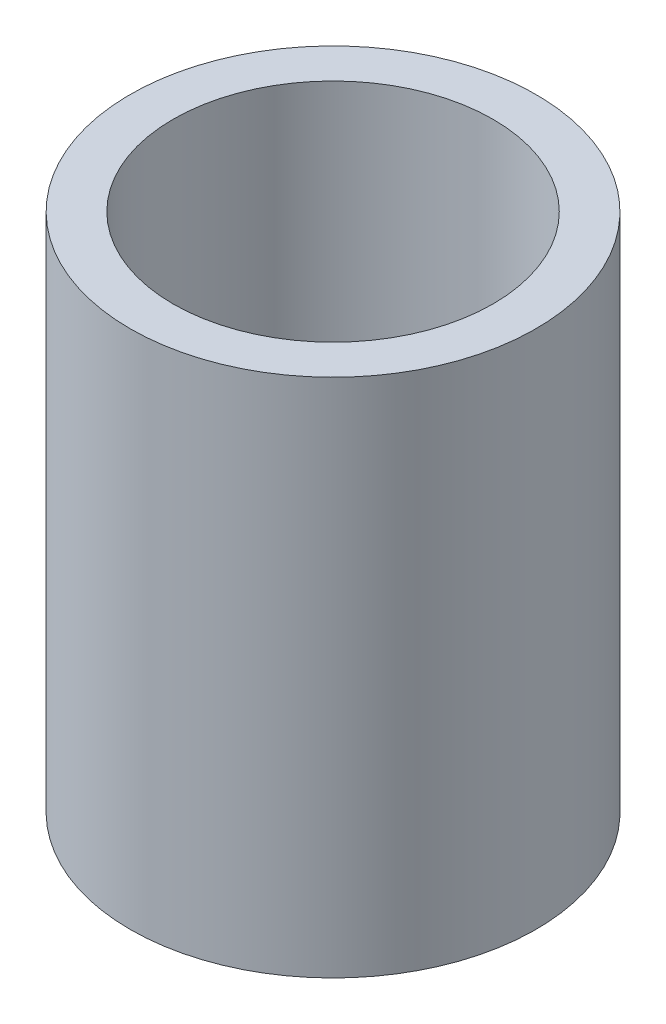
from build123d import *

# Parameters (mm, degrees)
SKETCH1_R           = 19.5
BOSS_EXTRUDE1_DEPTH = 50
G1_TAPPED_HOLE1_D   = 30.75


with BuildPart() as part:
    # Sketch1 → Boss-Extrude1 (new body)
    with BuildSketch(Plane(origin=(0, 0, 0), x_dir=(1, 0, 0), z_dir=(0, 1, 0))):
        with Locations(Location((0, 0, 0), (0, 0, 270))):
            Circle(SKETCH1_R)
    extrude(amount=BOSS_EXTRUDE1_DEPTH)

    # G1 Tapped Hole1 (through all)
    with Locations(Plane.ZX.offset(50)):
        with Locations((0, 0)):
            Hole(G1_TAPPED_HOLE1_D / 2)


solid = part.part
